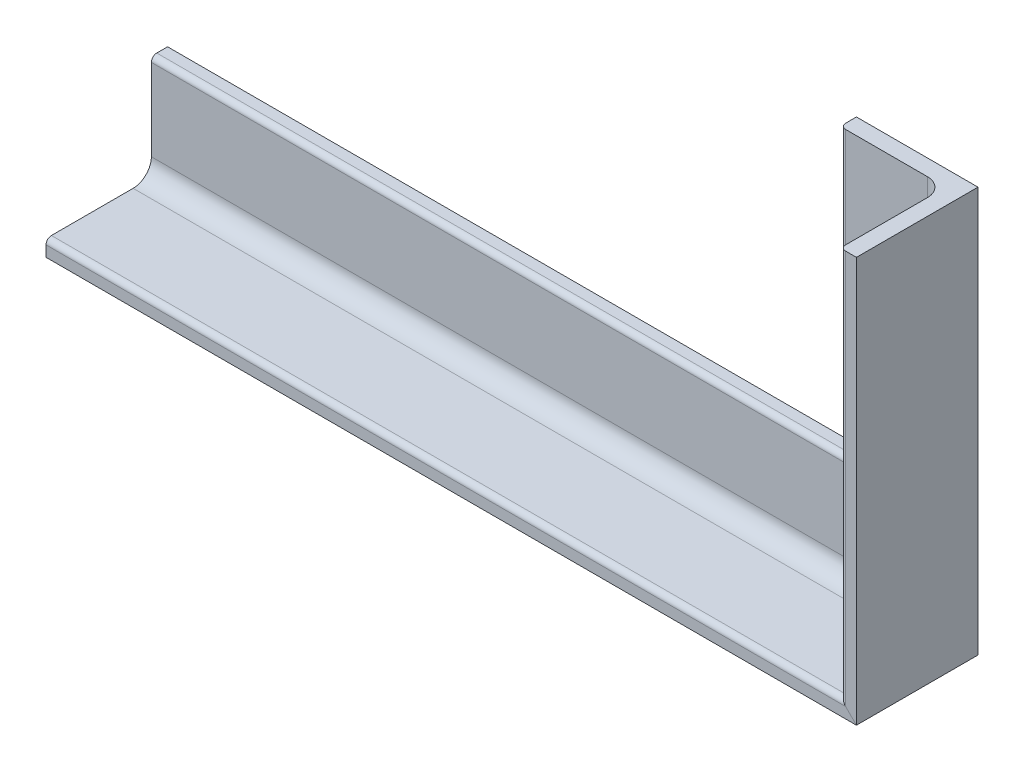
from build123d import *

# Parameters (mm, degrees)
GBT706_2008_030_4_1_DEPTH   = 243.426406871
GBT706_2008_030_4_1_2_DEPTH = 143.426406871


with BuildPart() as part:
    # Sketch12 → Gbt706-2008 热轧等边角钢 030×4(1) (new body)
    with BuildSketch(Plane.YZ):
        with BuildLine():
            Line((0, 0), (0, 30))
            Line((0, 30), (2.666666667, 30))
            ThreePointArc((2.666666667, 30), (3.609475708, 29.609475708), (4, 28.666666667))
            Line((4, 28.666666667), (4, 8.5))
            ThreePointArc((4, 8.5), (5.318019485, 5.318019485), (8.5, 4))
            Line((8.5, 4), (28.666666667, 4))
            ThreePointArc((28.666666667, 4), (29.609475708, 3.609475708), (30, 2.666666667))
            Line((30, 2.666666667), (30, 0))
            Line((30, 0), (0, 0))
        make_face()
    extrude(amount=GBT706_2008_030_4_1_DEPTH)

    # Gbt706-2008 热轧等边角钢 030×4(1) mitre 1
    split(bisect_by=Plane(origin=(200, 0, 0), x_dir=(0.707106781, -0.707106781, 0), z_dir=(-0.707106781, -0.707106781, 0)), keep=Keep.TOP)


with BuildPart() as body_2:
    # Sketch12 on segment 2 (carried to segment 2) → Gbt706-2008 _ 030_4_1 2 (new body)
    with BuildSketch(Plane(origin=(200, -43.426406871, 0), x_dir=(-1, 0, 0), z_dir=(0, 1, 0))):
        with BuildLine():
            Line((0, 0), (0, 30))
            Line((0, 30), (2.666666667, 30))
            ThreePointArc((2.666666667, 30), (3.609475708, 29.609475708), (4, 28.666666667))
            Line((4, 28.666666667), (4, 8.5))
            ThreePointArc((4, 8.5), (5.318019485, 5.318019485), (8.5, 4))
            Line((8.5, 4), (28.666666667, 4))
            ThreePointArc((28.666666667, 4), (29.609475708, 3.609475708), (30, 2.666666667))
            Line((30, 2.666666667), (30, 0))
            Line((30, 0), (0, 0))
        make_face()
    extrude(amount=GBT706_2008_030_4_1_2_DEPTH)

    # Gbt706-2008 _ 030_4_1 2 mitre 1
    split(bisect_by=Plane(origin=(200, 0, 0), x_dir=(-0.707106781, 0.707106781, 0), z_dir=(0.707106781, 0.707106781, 0)), keep=Keep.TOP)


solid = Compound([part.part, body_2.part])
